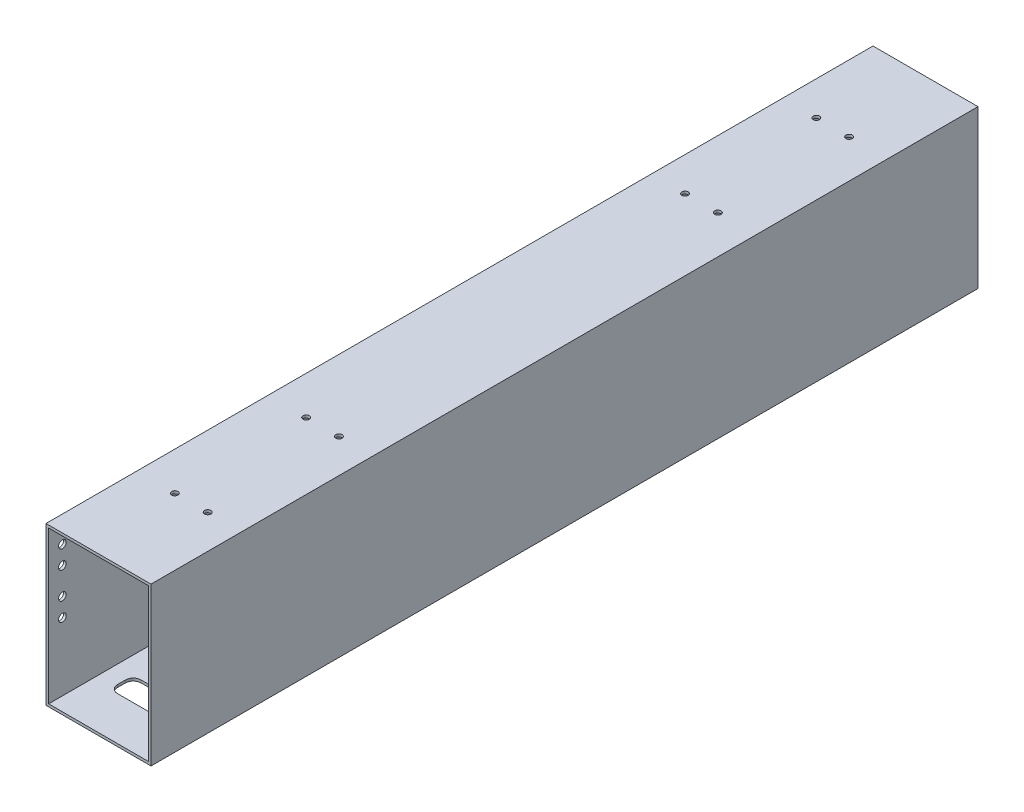
SolidWorks part; units mm, degrees
material "6061Al"
ref_plane "前视基准面" through (0, 0, 0) normal (0, 0, 1) x (1, 0, 0)
ref_plane "上视基准面" through (0, 0, 0) normal (0, 1, 0) x (1, 0, 0)
ref_plane "右视基准面" through (0, 0, 0) normal (1, 0, 0) x (0, 0, -1)
sketch "草图1" plane through (0, 0, 0) normal (0, 0, 1) x (1, 0, 0)
  line L1 (-40, -60) -> (40, -60)
  line L2 (-40, -60) -> (-40, 60)
  line L3 (-40, 60) -> (40, 60)
  line L4 (40, -60) -> (40, 60)
  line L5 (-40, -60) -> (40, 60) construction
  line L6 (-40, 60) -> (40, -60) construction
  point P0 (0, 0)
  dimension "D1" = 80
  dimension "D2" = 120
extrude "拉伸-薄壁1" add sketch "草图1" along normal mid plane 630 thin thin type one direction reverse wall 2
sketch "草图3" plane through (0, 0, 315) normal (0, 0, 1) x (1, 0, 0)
  line L0 (-40, -60) -> (40, -60) construction
  line L1 (-38, -58) -> (38, -58)
  line L2 (-38, -58) -> (-38, -60)
  line L3 (-38, -60) -> (38, -60)
  line L4 (38, -58) -> (38, -60)
  line L6 (38, -58) -> (38, 58) construction
sketch "草图4" plane through (-40, 0, 0) normal (-1, 0, 0) x (0, 0, 1)
  line L0 (315, -60) -> (-315, -60) construction
  circle A2 centre (0, -20) radius 25
  dimension "D1" = 50
  dimension "D2" = 40
extrude "切除-拉伸2" cut sketch "草图4" against normal up to next
hole_wizard "M5 间隙孔1" positions "草图7" profile "草图8" hole size "M5" standard "ISO"
sketch "草图7" plane through (-40, 0, 0) normal (-1, 0, 0) x (0, 0, 1)
  line L0 (0, 0) -> (0, -123.9236) construction
  line L1 (304.5, 28) -> (304.5, -6.39) construction
  line L2 (-304.5, 28) -> (-304.5, -6.39) construction
  line L5 (315, 60) -> (315, -60) construction
  line L6 (315, 60) -> (-315, 60) construction
  point P0 (304.5, 42)
  point P3 (304.5, 28)
  point P17 (304.5, 7.61)
  point P18 (304.5, -6.39)
  point P23 (-304.5, -6.39)
  point P24 (-304.5, 7.61)
  point P25 (-304.5, 28)
  point P26 (-304.5, 42)
  dimension "D2" = 14
  dimension "D3" = 304.5
  dimension "D4" = 14
  dimension "D5" = 20.39
  dimension "D6" = 10.5
  dimension "D7" = 18
  dimension "D1" = 2
sketch "草图8" plane through (-40, 42, 304.5) normal (0, 1, 0) x (0, 0, 1)
  line L0 (0, 0) -> (0, 2)
  line L1 (0, 2) -> (2.9, 2)
  line L2 (2.9, 2) -> (2.9, 0)
  line L5 (2.9, 0) -> (0, 0)
  line L11 (0, -6.35) -> (0, 107.95) construction
  dimension "通孔孔直径" = 5.8
  dimension "通孔孔深度" = 2
hole_wizard "M4 间隙孔1" positions "草图9" profile "草图10" hole size "M4" standard "ISO"
sketch "草图9" plane through (0, 60, 0) normal (0, 1, 0) x (1, 0, 0)
  line L1 (0, 0) -> (137.2059, 0) construction
  line L2 (-40, -315) -> (-40, 315) construction
  point P0 (-14.175, 246)
  point P3 (10.825, 246)
  point P6 (-14.175, 146)
  point P9 (10.825, 146)
  point P24 (-10.825, -146)
  point P27 (14.175, -146)
  point P30 (-10.825, -246)
  point P33 (14.175, -246)
  dimension "D1" = 25.825
  dimension "D2" = 100
  dimension "D3" = 50.825
  dimension "D4" = 100
  dimension "D5" = 29.175
  dimension "D6" = 246
  dimension "D7" = 25
  dimension "D8" = 246
sketch "草图10" plane through (-14.175, 60, -246) normal (1, 0, 0) x (0, 0, 1)
  line L0 (0, 0) -> (0, 2)
  line L1 (0, 2) -> (2.4, 2)
  line L2 (2.4, 2) -> (2.4, 0)
  line L5 (2.4, 0) -> (0, 0)
  line L11 (0, -6.35) -> (0, 107.95) construction
  dimension "通孔孔直径" = 4.8
  dimension "通孔孔深度" = 2
sketch "草图15" plane through (0, -60, 0) normal (0, -1, 0) x (1, 0, 0)
  line L0 (0.475, -275) -> (0.475, -271) construction
  line L1 (-19.025, -275) -> (19.975, -275) construction
  line L2 (19.975, -271) -> (-19.025, -271) construction
  line L3 (1.975, -160.4169) -> (1.975, -234.9622) construction
  line L4 (25.475, -282) -> (-24.525, -282)
  line L5 (25.475, -282) -> (25.475, -264)
  line L6 (25.475, -264) -> (-24.525, -264)
  line L7 (-24.525, -282) -> (-24.525, -264)
  line L8 (25.475, -282) -> (-24.525, -264) construction
  line L9 (25.475, -264) -> (-24.525, -282) construction
  line L11 (0, 0) -> (190.9688, 0) construction
  line L12 (-28.025, -209) -> (31.975, -209)
  line L13 (-28.025, -209) -> (-28.025, -134)
  line L14 (-28.025, -134) -> (31.975, -134)
  line L15 (31.975, -209) -> (31.975, -134)
  line L16 (25.475, 264) -> (-24.525, 282) construction
  line L17 (25.475, 282) -> (-24.525, 264) construction
  line L18 (1.975, 160.4169) -> (1.975, 234.9622) construction
  line L19 (0.475, 275) -> (0.475, 271) construction
  line L20 (31.975, 209) -> (31.975, 134)
  line L21 (-28.025, 134) -> (31.975, 134)
  line L22 (-28.025, 209) -> (-28.025, 134)
  line L23 (-28.025, 209) -> (31.975, 209)
  line L24 (-24.525, 282) -> (-24.525, 264)
  line L25 (25.475, 264) -> (-24.525, 264)
  line L26 (25.475, 282) -> (25.475, 264)
  line L27 (25.475, 282) -> (-24.525, 282)
  point P6 (0.475, -273)
  point P33 (0.475, 273)
  dimension "D1" = 18
  dimension "D2" = 50
  dimension "D3" = 130
  dimension "D4" = 75
  dimension "D5" = 60
extrude "切除-拉伸3" cut sketch "草图15" against normal up to next
fillet "圆角1" radius 6 16 edges at (-28.025, -59, -209) (-28.025, -59, -134) (31.975, -59, -134) (31.975, -59, -209) (25.475, -59, 282) (25.475, -59, 264) (-24.525, -59, 264) (-24.525, -59, 282) (-28.025, -59, 209) (31.975, -59, 209) (31.975, -59, 134) (-28.025, -59, 134) (-24.525, -59, -264) (25.475, -59, -264) (25.475, -59, -282) (-24.525, -59, -282)
